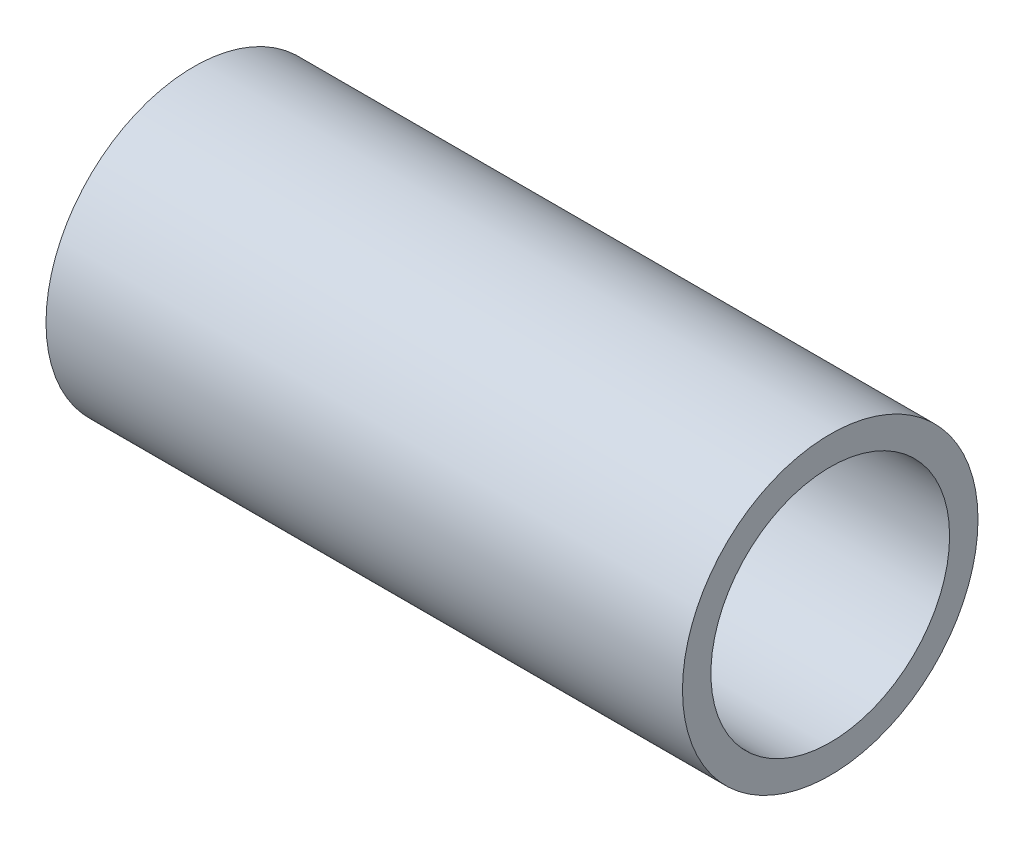
from build123d import *

# Parameters (mm, degrees)
SKETCH1_R           = 13
SKETCH1_R_2         = 10.5
BOSS_EXTRUDE1_DEPTH = 56


with BuildPart() as part:
    # Sketch1 → Boss-Extrude1 (new body)
    with BuildSketch(Plane(origin=(0, 0, 0), x_dir=(0, 0, -1), z_dir=(1, 0, 0))):
        Circle(SKETCH1_R)
        Circle(SKETCH1_R_2, mode=Mode.SUBTRACT)
    extrude(amount=BOSS_EXTRUDE1_DEPTH)


solid = part.part
